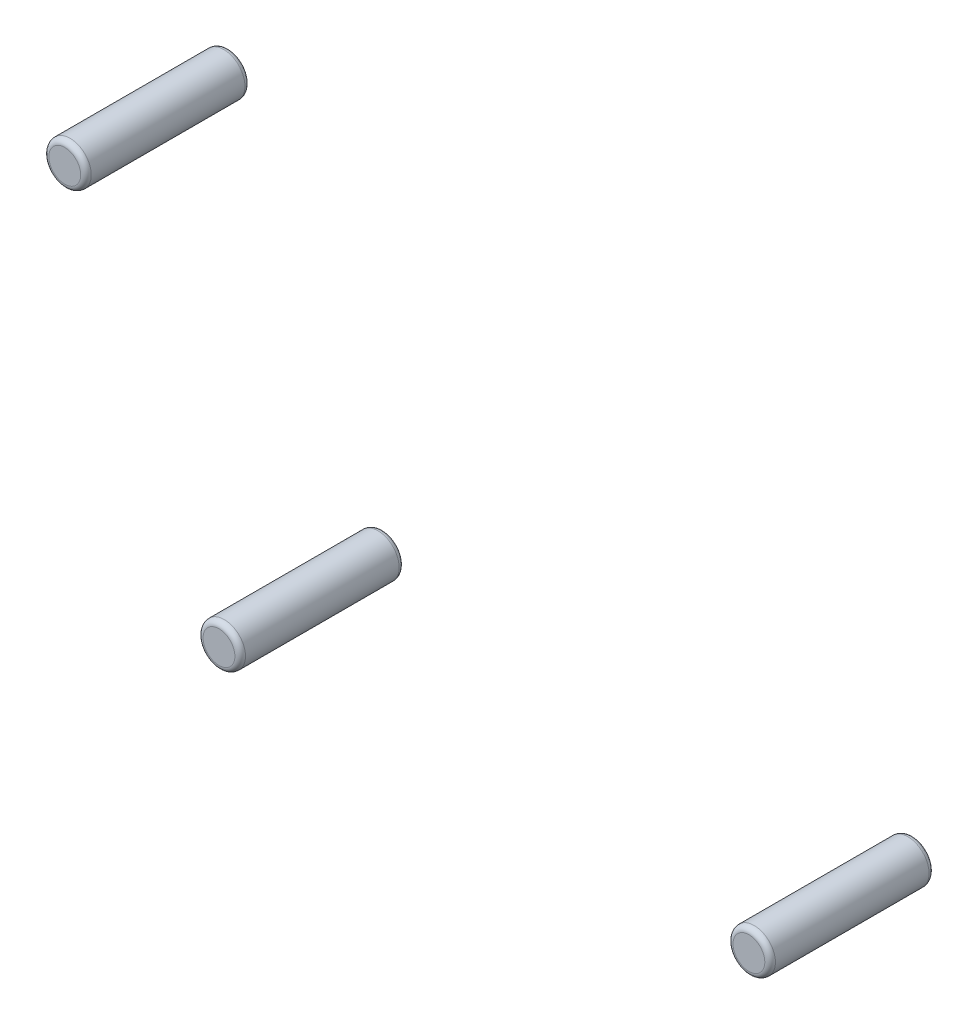
SolidWorks part; units mm, degrees
ref_plane "Front Plane" through (0, 0, 0) normal (0, 0, 1) x (1, 0, 0)
ref_plane "Top Plane" through (0, 0, 0) normal (0, 1, 0) x (1, 0, 0)
ref_plane "Right Plane" through (0, 0, 0) normal (1, 0, 0) x (0, 0, -1)
sketch "Sketch1" plane through (0, 0, 0) normal (0, 0, 1) x (1, 0, 0)
  circle A0 centre (-79.1, 0) radius 4 construction
  circle A1 centre (-79.1, 0) radius 4
  circle A2 centre (-50, -64.1) radius 4
  circle A3 centre (50, -64.1) radius 4
  dimension "D1" = 8
  dimension "D2" = 8
  dimension "D3" = 8
extrude "Boss-Extrude1" add sketch "Sketch1" along normal blind 26 and the other way up to surface (5 mm away)
fillet "Fillet1" radius 1 2 edges at (-75.1, 0, 26) (-83.1, 0, -5)
fillet "Fillet2" radius 1 2 edges at (-46, -64.1, 26) (-54, -64.1, -5)
fillet "Fillet3" radius 1 2 edges at (46, -64.1, -5) (54, -64.1, 26)
